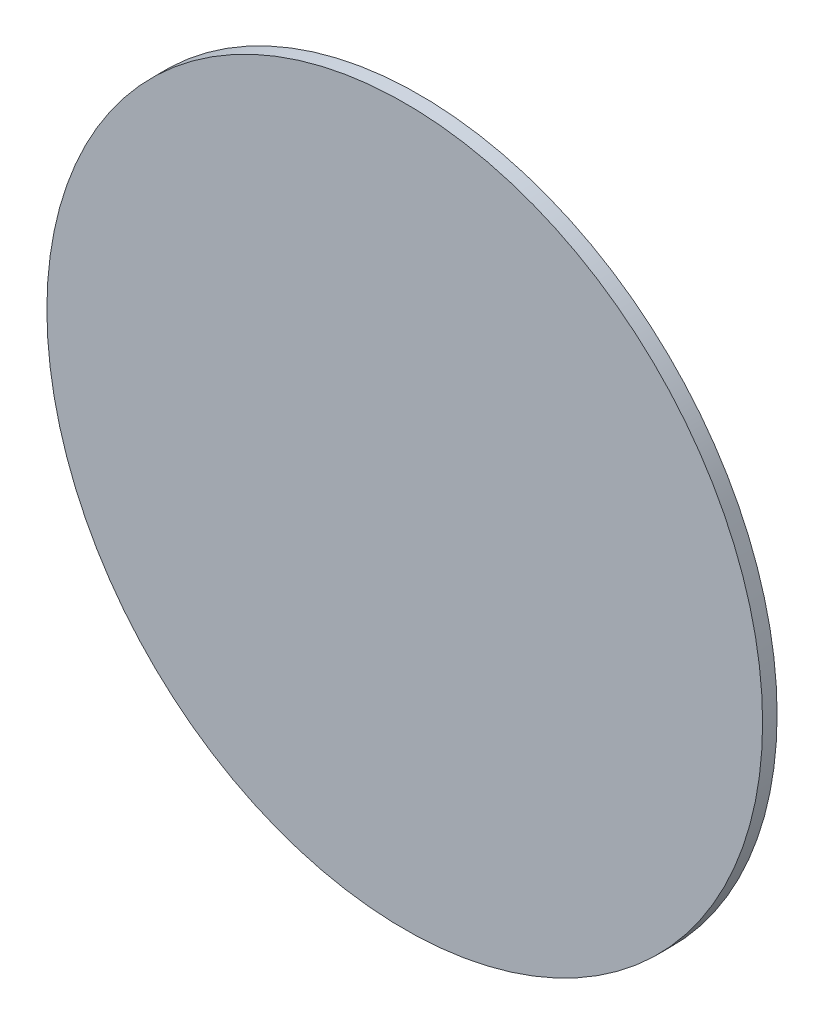
SolidWorks part; units mm, degrees
material "玻璃"
ref_plane "Front plane" through (0, 0, 0) normal (0, 0, 1) x (1, 0, 0)
ref_plane "Top plane" through (0, 0, 0) normal (0, 1, 0) x (1, 0, 0)
ref_plane "Right plane" through (0, 0, 0) normal (1, 0, 0) x (0, 0, -1)
sketch "Sketch 1" plane through (0, 0, 0) normal (0, 0, 1) x (1, 0, 0)
  circle A0 centre (0, 0) radius 74
  dimension "D1" = 148
extrude "Boss-Extrude 1" add sketch "Sketch 1" along normal blind 3
